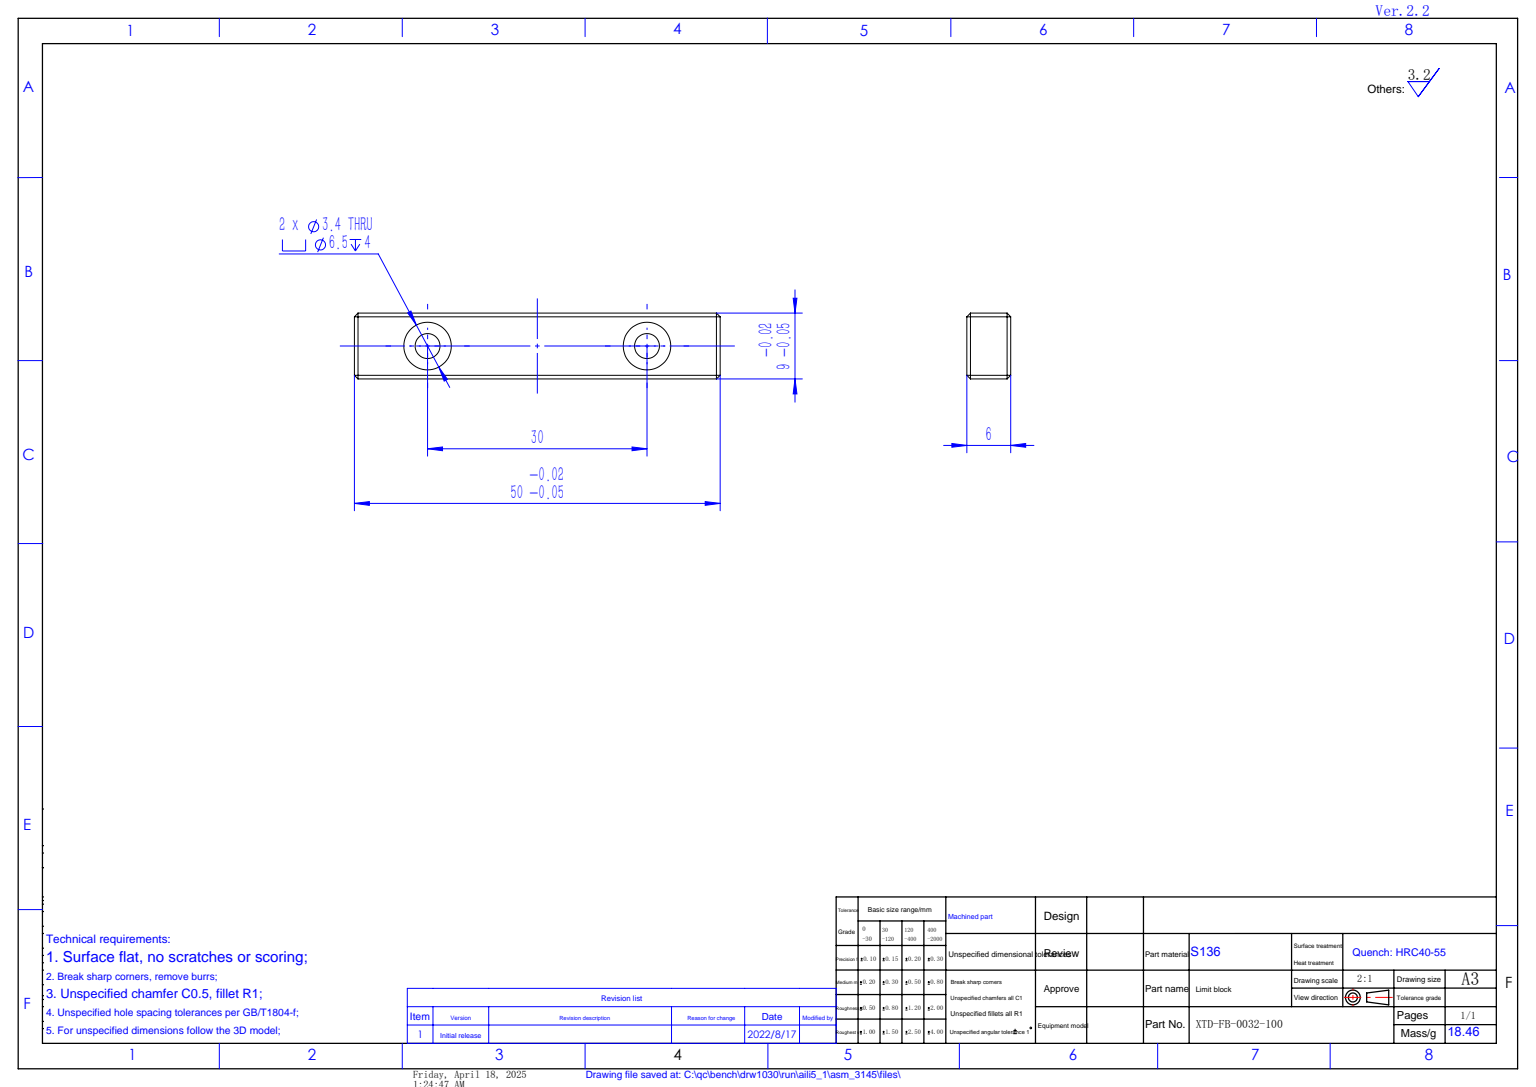
from build123d import *

# Parameters (mm, degrees)
SKETCH_1_W                   = 50
SKETCH_1_H                   = 9
EXTRUDE_1_DEPTH              = 6
CHAMFER_1_SIZE               = 0.5
HOLE_WIZARD_M3_1_D           = 3.4
HOLE_WIZARD_M3_1_CBORE_D     = 6.5
HOLE_WIZARD_M3_1_CBORE_DEPTH = 4


with BuildPart() as part:
    # 草图1 → 凸台-拉伸1 (new body)
    with BuildSketch(Plane(origin=(0, 0, 0), x_dir=(1, 0, 0), z_dir=(0, 1, 0))):
        Rectangle(SKETCH_1_W, SKETCH_1_H)
    extrude(amount=EXTRUDE_1_DEPTH)

    # 倒角1
    chamfer_1_edges = [part.edges().sort_by_distance(p)[0] for p in [
        (25, 6, 0),
        (0, 6, -4.5),
        (-25, 6, 0),
        (0, 0, -4.5),
        (25, 0, 0),
        (0, 0, 4.5),
        (-25, 0, 0),
        (-25, 3, -4.5),
        (25, 3, -4.5),
        (25, 3, 4.5),
        (-25, 3, 4.5),
        (0, 6, 4.5),
    ]]
    chamfer(chamfer_1_edges, length=CHAMFER_1_SIZE)

    # M3 六角凹头螺钉的柱形沉头孔1 (through all)
    with Locations(Plane(origin=(0, 6, 0), x_dir=(1, 0, 0), z_dir=(0, 1, 0))):
        with Locations((-15, 0), (15, 0)):
            CounterBoreHole(HOLE_WIZARD_M3_1_D / 2, HOLE_WIZARD_M3_1_CBORE_D / 2, HOLE_WIZARD_M3_1_CBORE_DEPTH)


solid = part.part
